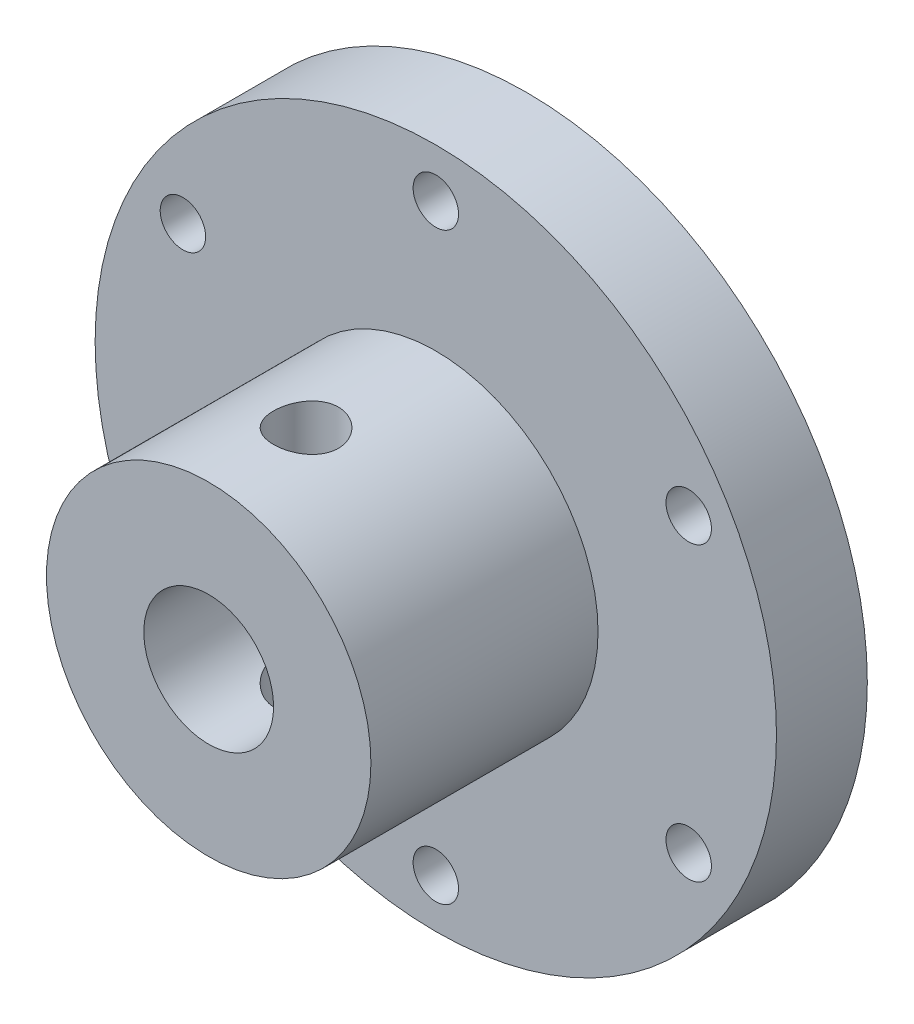
from build123d import *

# Parameters (mm, degrees)
SKETCH1_R               = 52.5
SKETCH1_R_2             = 3.5
BOSS_EXTRUDE1_DEPTH     = 14
SKETCH2_R               = 25
SKETCH2_R_2             = 10
BOSS_EXTRUDE2_DEPTH     = 35
CUT_EXTRUDE1_DEPTH      = 89.95785519
CUT_EXTRUDE1_DEPTH_BACK = 89.95785519
SKETCH3_R               = 5


with BuildPart() as part:
    # Sketch1 → Boss-Extrude1 (new body)
    with BuildSketch(Plane.XY):
        Circle(SKETCH1_R)
        with Locations((0, 45)):
            Circle(SKETCH1_R_2, mode=Mode.SUBTRACT)
        with Locations((38.97114317, 22.5)):
            Circle(SKETCH1_R_2, mode=Mode.SUBTRACT)
        with Locations((38.97114317, -22.5)):
            Circle(SKETCH1_R_2, mode=Mode.SUBTRACT)
        with Locations((0, -45)):
            Circle(SKETCH1_R_2, mode=Mode.SUBTRACT)
        with Locations((-38.97114317, -22.5)):
            Circle(SKETCH1_R_2, mode=Mode.SUBTRACT)
        with Locations((-38.97114317, 22.5)):
            Circle(SKETCH1_R_2, mode=Mode.SUBTRACT)
    extrude(amount=BOSS_EXTRUDE1_DEPTH)

    # Sketch2 → Boss-Extrude2 (add)
    with BuildSketch(Plane.XY.offset(14)):
        Circle(SKETCH2_R)
        Circle(SKETCH2_R_2, mode=Mode.SUBTRACT)
    extrude(amount=BOSS_EXTRUDE2_DEPTH)

    # Sketch3 → Cut-Extrude1 (cut, two sides: drawn at the far end of the back side and taken through both)
    with BuildSketch(Plane(origin=(0, 0, 0), x_dir=(1, 0, 0), z_dir=(0, 1, 0)).offset(-CUT_EXTRUDE1_DEPTH_BACK)):
        with Locations(Location((0, -34, 0), (0, 0, 270))):
            Circle(SKETCH3_R)
    extrude(amount=CUT_EXTRUDE1_DEPTH + CUT_EXTRUDE1_DEPTH_BACK, mode=Mode.SUBTRACT)


solid = part.part
